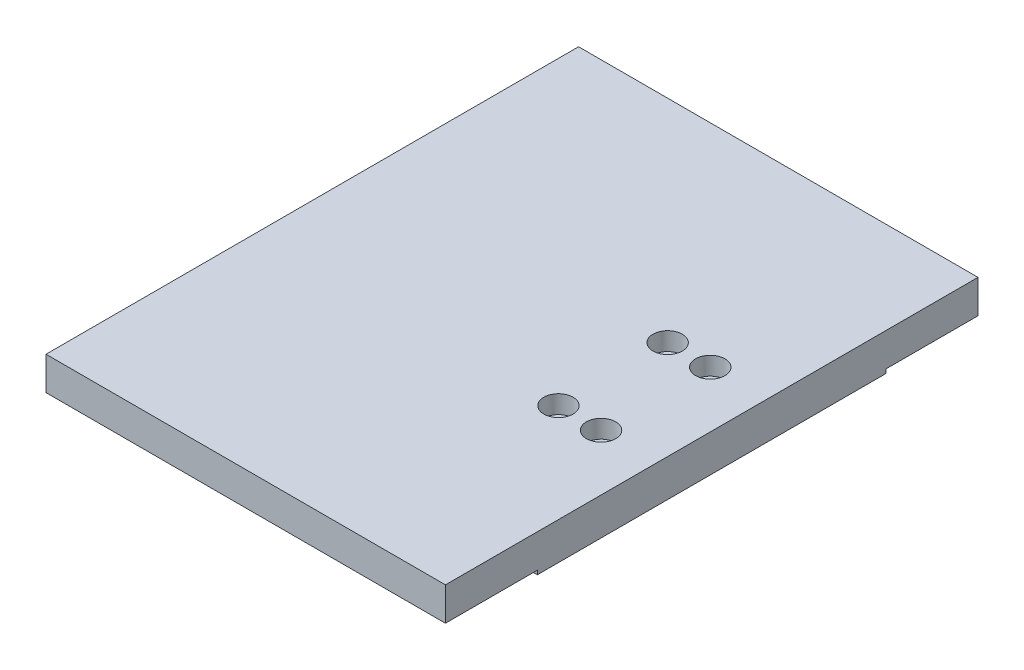
SolidWorks part; units mm, degrees
material "6061 铝合金"
ref_plane "前视基准面" through (0, 0, 0) normal (0, 0, 1) x (1, 0, 0)
ref_plane "上视基准面" through (0, 0, 0) normal (0, 1, 0) x (1, 0, 0)
ref_plane "右视基准面" through (0, 0, 0) normal (1, 0, 0) x (0, 0, -1)
sketch "草图1" plane through (0, 0, 0) normal (0, 1, 0) x (1, 0, 0)
  line L1 (-75, -100) -> (75, -100)
  line L2 (-75, -100) -> (-75, 100)
  line L3 (-75, 100) -> (75, 100)
  line L4 (75, -100) -> (75, 100)
  line L5 (-75, -100) -> (75, 100) construction
  line L6 (-75, 100) -> (75, -100) construction
  point P0 (0, 0)
  dimension "D1" = 200
  dimension "D2" = 150
extrude "凸台-拉伸1" add sketch "草图1" along normal blind 14
sketch "草图2" plane through (0, 0, 0) normal (0, -1, 0) x (1, 0, 0)
  line L0 (75, 100) -> (75, -100) construction
  line L1 (-75, 100) -> (75, 100)
  line L2 (-75, 100) -> (-75, 65.5)
  line L3 (-75, 65.5) -> (75, 65.5)
  line L4 (75, 100) -> (75, 65.5)
  line L6 (-75, -100) -> (75, -100)
  line L7 (-75, -100) -> (-75, -65.5)
  line L8 (-75, -65.5) -> (75, -65.5)
  line L9 (75, -100) -> (75, -65.5)
  dimension "D1" = 131
extrude "切除-拉伸1" cut sketch "草图2" against normal blind 1.5
hole_wizard "打孔尺寸(%根据)内六角圆柱头螺钉的类型1" positions "3D草图1" profile "草图3" counterbore size "M6" standard "GB" end condition up to next
sketch3d "3D草图1"
  line L0 (75, 14, 100) -> (75, 14, -100) construction
  line L1 (75, 14, 0) -> (-75, 14, 0)
  line L2 (-75, 14, -100) -> (-75, 14, 100) construction
  point P0 (37.95, 14, 20.5)
  point P2 (37.95, 14, -20.5)
  point P4 (53.95, 14, 20.5)
  point P6 (53.95, 14, -20.5)
  dimension "D1" = 41
  dimension "D2" = 16
  dimension "D3" = 21.05
  dimension "D4" = 20.5
sketch "草图3" plane through (37.95, 14, 20.5) normal (1, 0, 0) x (0, 0, 1)
  line L0 (0, 0) -> (0, 14)
  line L1 (0, 14) -> (3.3, 14)
  line L3 (3.3, 14) -> (3.3, 6.8)
  line L4 (3.3, 6.8) -> (5.5, 6.8)
  line L5 (5.5, 6.8) -> (5.5, 0)
  line L7 (5.5, 0) -> (0, 0)
  line L11 (0, -6.35) -> (0, 107.95) construction
  dimension "通孔孔直径" = 6.6
  dimension "通孔孔深度" = 14
  dimension "柱形沉头孔直径" = 11
  dimension "柱形沉头孔深度" = 6.8
sketch "草图4" plane through (0, 14, 0) normal (0, 1, 0) x (1, 0, 0)
  line L0 (-75, -100) -> (75, -100) construction
  line L1 (10, -100) -> (-4.5, -100)
  line L2 (10, -100) -> (10, 100)
  line L3 (10, 100) -> (-4.5, 100)
  line L4 (-4.5, -100) -> (-4.5, 100)
  line L5 (75, 100) -> (-75, 100) construction
  line L6 (75, -100) -> (75, 100) construction
  dimension "D1" = 14.5
  dimension "D2" = 65
extrude "切除-拉伸2" [suppressed] cut sketch "草图4" against normal blind 1.5
